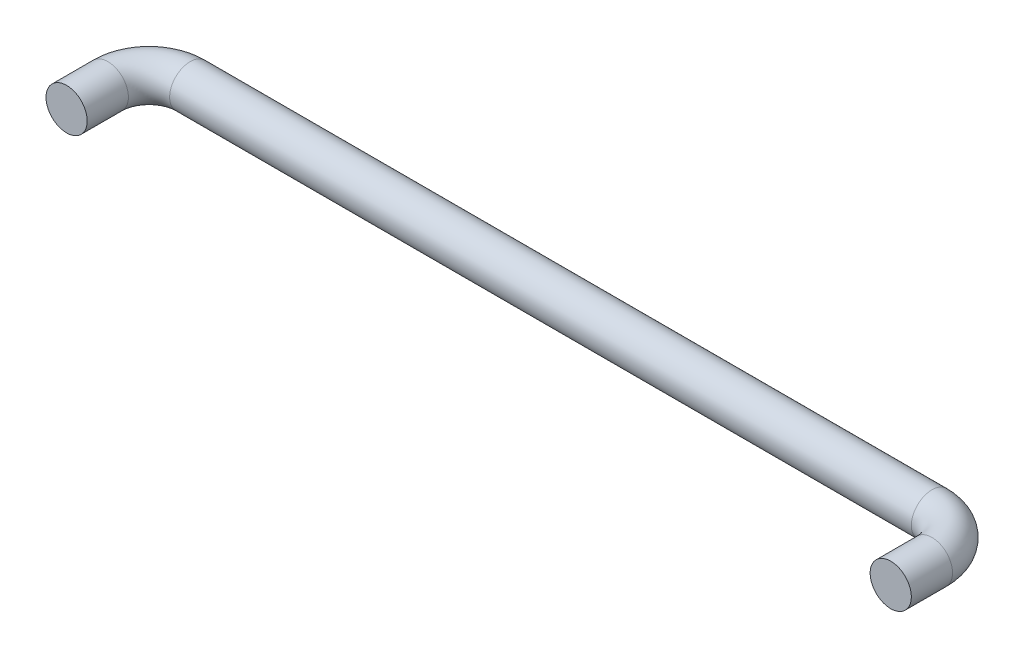
SolidWorks part; units mm, degrees
ref_plane "Front Plane" through (0, 0, 0) normal (0, 0, 1) x (1, 0, 0)
ref_plane "Top Plane" through (0, 0, 0) normal (0, 1, 0) x (1, 0, 0)
ref_plane "Right Plane" through (0, 0, 0) normal (1, 0, 0) x (0, 0, -1)
sketch "Sketch1" plane through (0, 0, 0) normal (0, 1, 0) x (1, 0, 0)
  line L0 (5, 0) -> (95, 0)
  line L1 (0, -5) -> (0, -10)
  line L2 (100, -5) -> (100, -10)
  arc A0 (95, 0) -> (100, -5) centre (95, -5) cw
  arc A1 (5, 0) -> (0, -5) centre (5, -5) ccw
  point P7 (100, 0)
  point P10 (0, 0)
  dimension "D4" = 5
  dimension "D1" = 100
  dimension "D2" = 10
  dimension "D3" = 10
sweep "Sweep1" add path "Sketch1" circular profile diameter 5 parameters "D3"=5
